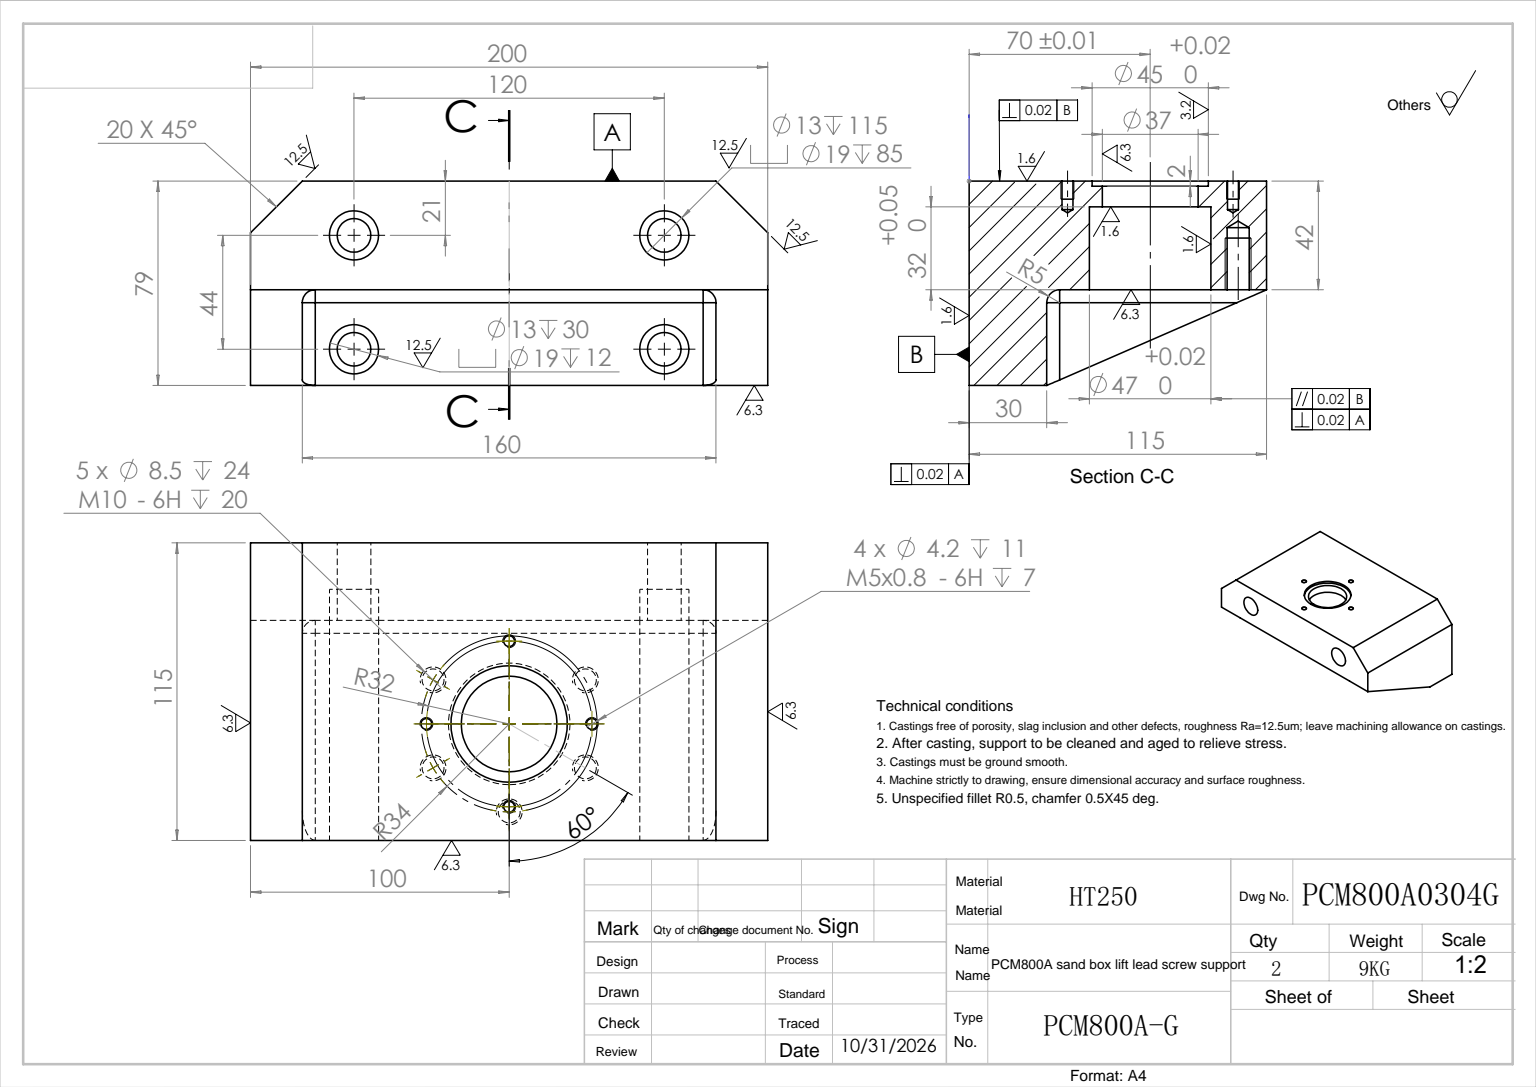
SolidWorks part; units mm, degrees
ref_plane "前视基准面" through (0, 0, 0) normal (0, 0, 1) x (1, 0, 0)
ref_plane "上视基准面" through (0, 0, 0) normal (0, 1, 0) x (1, 0, 0)
ref_plane "右视基准面" through (0, 0, 0) normal (1, 0, 0) x (0, 0, -1)
sketch "草图1" plane through (0, 0, 0) normal (0, 0, 1) x (1, 0, 0)
  line L0 (80, 0) -> (-80, 0)
  line L1 (-80, 0) -> (-100, -20)
  line L2 (-100, -20) -> (-100, -42)
  line L3 (-100, -42) -> (100, -42)
  line L4 (0, 0) -> (0, -99.4201) construction
  line L5 (100, -20) -> (100, -42)
  line L6 (80, 0) -> (100, -20)
  point P8 (0, -42)
  dimension "D1" = 80
  dimension "D2" = 100
  dimension "D3" = 42
extrude "拉伸1" add sketch "草图1" along normal blind 115
sketch "草图2" plane through (0, 0, 0) normal (0, 0, 1) x (1, 0, 0)
  line L1 (-100, -42) -> (100, -42)
  line L2 (-100, -42) -> (-100, -79)
  line L3 (-100, -79) -> (100, -79)
  line L4 (100, -42) -> (100, -79)
  dimension "D1" = 37
  dimension "D2" = 200
extrude "拉伸2" add sketch "草图2" along normal blind 30
sketch "草图3" plane through (-100, 0, 0) normal (-1, 0, 0) x (0, 0, 1)
  line L0 (30, -79) -> (30, -42)
  line L1 (30, -42) -> (115, -42)
  line L2 (115, -42) -> (30, -79)
  line L3 (30, -79) -> (30.1902, -80.1907)
  line M3 (30, -79) -> (30, -42)
  line M4 (30, -42) -> (115, -42)
extrude "拉伸3" add sketch "草图3" against normal blind 20 contours L2 M4 M3
mirror "镜向1" about plane through (0, 0, 0) normal (1, 0, 0) of "拉伸3"
sketch "草图4" plane through (0, 0, 0) normal (0, 1, 0) x (1, 0, 0)
  line L0 (0, 0) -> (0, -115) construction
  line L1 (80, -115) -> (-80, -115) construction
  line L2 (-80, -70) -> (77.4671, -70) construction
  line L3 (-80, -115) -> (-80, 0) construction
  line L4 (80, 0) -> (-80, 0) construction
  circle A0 centre (0, -70) radius 22.5
  dimension "D1" = 70
extrude "切除-拉伸1" cut sketch "草图4" against normal blind 2
sketch "草图5" plane through (0, -2, 0) normal (0, 1, 0) x (1, 0, 0)
  circle A0 centre (0, -70) radius 18.5
extrude "切除-拉伸2" cut sketch "草图5" against normal blind 8
sketch "草图6" plane through (0, -10, 0) normal (0, 1, 0) x (1, 0, 0)
  circle A0 centre (0, -70) radius 23.5
extrude "切除-拉伸3" cut sketch "草图6" against normal up to next
sketch "草图7" plane through (0, 0, 115) normal (0, 0, 1) x (1, 0, 0)
  line L0 (-97.6106, -21) -> (86.4674, -21) construction
  line L1 (-60, -4.6416) -> (-60, -38.7142) construction
  line L2 (60, 0) -> (60, -41.0715) construction
  line L3 (80, 0) -> (-80, 0) construction
  line L4 (100, -42) -> (100, -20) construction
  circle A0 centre (60, -21) radius 9.5
  circle A1 centre (-60, -21) radius 9.5
  point P8 (100, -31)
  dimension "D1" = 21
  dimension "D2" = 120
  dimension "D3" = 40
extrude "切除-拉伸4" cut sketch "草图7" against normal blind 85
sketch "草图8" plane through (0, 0, 30) normal (0, 0, 1) x (1, 0, 0)
  circle A0 centre (-60, -21) radius 6.5
  circle A1 centre (60, -21) radius 6.5
extrude "切除-拉伸5" cut sketch "草图8" against normal through all
sketch "草图9" plane through (0, -42, 0) normal (0, -1, 0) x (1, 0, 0)
  line L0 (0, 70) -> (-45.0727, 96.0227) construction
  line L1 (0, 70) -> (57.5733, 103.24) construction
  line L2 (0, 70) -> (-44.9871, 44.0267) construction
  line L3 (0, 70) -> (46.1729, 43.3421) construction
  line L4 (0, 70) -> (0, 106.5) construction
  circle A0 centre (0, 70) radius 34 construction
  circle A1 centre (0, 104) radius 2.5
  circle A2 centre (29.4449, 87) radius 2.5
  circle A3 centre (29.4449, 53) radius 2.5
  circle A4 centre (-29.4449, 87) radius 2.5
  circle A5 centre (-29.4449, 53) radius 2.5
  dimension "D1" = 60
  dimension "D5" = 5
  dimension "D6" = 5
  dimension "D7" = 5
  dimension "D8" = 5
  dimension "D9" = 5
  dimension "D2" = 60
  dimension "D3" = 60
  dimension "D4" = 60
extrude "切除-拉伸6" cut sketch "草图9" against normal blind 10
fillet "圆角1" radius 5 5 edges at (-80, -60.5, 30) (80, -60.5, 30) (80, -42, 72.5) (-80, -42, 72.5)
sketch "草图10" plane through (0, 0, 0) normal (0, 1, 0) x (1, 0, 0)
  circle A0 centre (0, -70) radius 32 construction
  circle A1 centre (0, -38) radius 1
  circle A2 centre (32, -70) radius 1
  circle A3 centre (0, -102) radius 1
  circle A4 centre (-32, -70) radius 1
  dimension "D1" = 2
  dimension "D2" = 2
  dimension "D3" = 2
  dimension "D4" = 2
extrude "切除-拉伸7" cut sketch "草图10" against normal blind 5
hole_wizard "M5x0.8 螺纹孔1" positions "草图12" profile "草图11" tap size "M5x0.8" standard "Ansi Metric"
sketch "草图12" plane through (0, 0, 0) normal (0, 1, 0) x (-1, 0, 0)
  point P0 (0, 38)
  point P1 (-32, 70)
  point P3 (0, 102)
  point P5 (32, 70)
sketch "草图11" plane through (0, 0, 38) normal (1, 0, 0) x (0, 0, 1)
  line L0 (0, 0) -> (0, 12.2618)
  line L1 (0, 12.2618) -> (2.1, 11)
  line L2 (2.1, 11) -> (2.1, 0)
  line L5 (2.1, 0) -> (0, 0)
  line L10 (0, 12.2618) -> (-2.1, 11) construction
  line L11 (0, -6.35) -> (0, 107.95) construction
  dimension "螺纹孔钻头直径" = 4.2
  dimension "螺纹孔钻头深度" = 11
  dimension "导头角度" = 118
cosmetic thread "孔螺蚊线1" parameters "D1"=7, "D2"=5
cosmetic thread "孔螺蚊线2" parameters "D1"=7, "D2"=5
cosmetic thread "孔螺蚊线3" parameters "D1"=7, "D2"=5
cosmetic thread "孔螺蚊线4" parameters "D1"=7, "D2"=5
hole_wizard "M10 螺纹孔1" positions "草图14" profile "草图13" tap size "M10" standard "GB"
sketch "草图14" plane through (0, -42, 0) normal (0, -1, 0) x (1, 0, 0)
  point P0 (29.4449, 53)
  point P1 (29.4449, 87)
  point P3 (0, 104)
  point P5 (-29.4449, 87)
  point P7 (-29.4449, 53)
sketch "草图13" plane through (29.4449, -42, 53) normal (1, 0, 0) x (0, 0, -1)
  line L0 (0, 0) -> (0, 26.5537)
  line L1 (0, 26.5537) -> (4.25, 24)
  line L2 (4.25, 24) -> (4.25, 0)
  line L5 (4.25, 0) -> (0, 0)
  line L10 (0, 26.5537) -> (-4.25, 24) construction
  line L11 (0, -6.35) -> (0, 107.95) construction
  dimension "螺纹孔钻头直径" = 8.5
  dimension "螺纹孔钻头深度" = 24
  dimension "导头角度" = 118
cosmetic thread "孔螺蚊线5" parameters "D1"=20, "D2"=10
cosmetic thread "孔螺蚊线6" parameters "D1"=20, "D2"=10
cosmetic thread "孔螺蚊线7" parameters "D1"=20, "D2"=10
cosmetic thread "孔螺蚊线8" parameters "D1"=20, "D2"=10
cosmetic thread "孔螺蚊线9" parameters "D1"=20, "D2"=10
sketch "草图15" plane through (0, 0, 30) normal (0, 0, 1) x (1, 0, 0)
  line L0 (-60, -21) -> (-60, -106.69) construction
  circle A0 centre (-60, -65) radius 6.5
  circle A1 centre (60, -65) radius 6.5
  dimension "D1" = 13
  dimension "D2" = 13
  dimension "D3" = 120
  dimension "D4" = 44
extrude "切除-拉伸8" cut sketch "草图15" against normal blind 55
sketch "草图16" plane through (0, 0, 30) normal (0, 0, 1) x (1, 0, 0)
  circle A0 centre (-60, -65) radius 9.5
  circle A1 centre (60, -65) radius 9.5
  dimension "D1" = 19
  dimension "D2" = 19
extrude "切除-拉伸9" cut sketch "草图16" against normal blind 12
